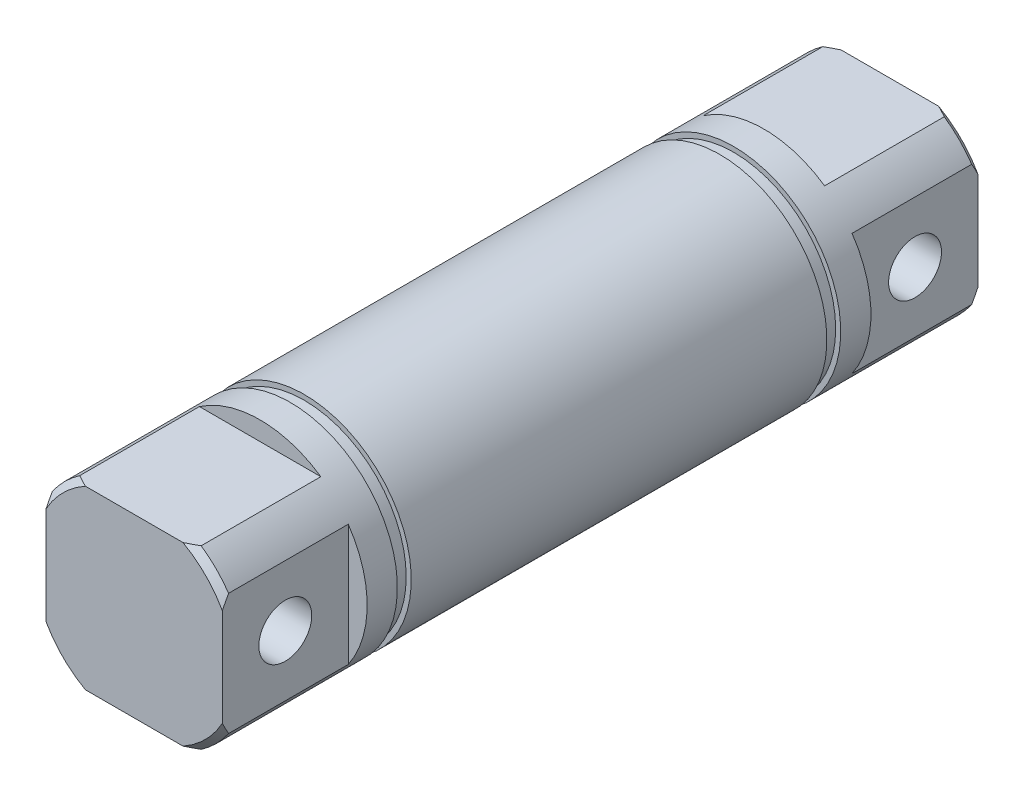
from build123d import *

# Parameters (mm, degrees)
SKETCH_1_R           = 8.5
EXTRUDE_1_DEPTH      = 30
SKETCH_4_OUTSIDE_W   = 31.928
SKETCH_4_OUTSIDE_H   = 31.928
SKETCH_4_OUTSIDE_W_2 = 14
SKETCH_4_OUTSIDE_H_2 = 14
CUT_EXTRUDE_1_DEPTH  = 10
HOLE_WIZARD_M5_1_D   = 4.2
CHAMFER_1_SIZE       = 0.5
SKETCH_7_W           = 0.4
SKETCH_7_H           = 1.1


with BuildPart() as part:
    # 草图1 → 凸台-拉伸1 (new, symmetric)
    with BuildSketch(Plane.XY):
        Circle(SKETCH_1_R)
    extrude(amount=EXTRUDE_1_DEPTH, both=True)

    # 草图4 outside → 切除-拉伸1 (cut)
    with BuildSketch(Plane.XY.offset(30)):
        Rectangle(SKETCH_4_OUTSIDE_W, SKETCH_4_OUTSIDE_H)
        Rectangle(SKETCH_4_OUTSIDE_W_2, SKETCH_4_OUTSIDE_H_2, mode=Mode.SUBTRACT)
    cut_extrude_1 = extrude(amount=-CUT_EXTRUDE_1_DEPTH, mode=Mode.SUBTRACT)

    # M5 螺纹孔1 (through all)
    with Locations(Plane(origin=(7, 0, 0), x_dir=(0, 0, -1), z_dir=(1, 0, 0))):
        with Locations((-25, 0)):
            hole_wizard_m5_1 = Hole(HOLE_WIZARD_M5_1_D / 2)

    # 镜向1: 切除-拉伸1, M5 螺纹孔1 across plane
    add(cut_extrude_1.mirror(Plane.XY), mode=Mode.SUBTRACT)
    add(hole_wizard_m5_1.mirror(Plane.XY), mode=Mode.SUBTRACT)

    # 倒角1
    chamfer_1_edges = [part.edges().sort_by_distance(p)[0] for p in [
        (6.01040764, 6.01040764, -30),
        (6.01040764, 6.01040764, 30),
        (-6.01040764, 6.01040764, 30),
        (-6.01040764, 6.01040764, -30),
        (-6.01040764, -6.01040764, -30),
        (6.01040764, -6.01040764, -30),
        (-6.01040764, -6.01040764, 30),
        (6.01040764, -6.01040764, 30),
    ]]
    chamfer(chamfer_1_edges, length=CHAMFER_1_SIZE)

    # 草图7 → 切除-旋转1 (revolve, cut)
    with BuildSketch(Plane(origin=(0, 0, 0), x_dir=(1, 0, 0), z_dir=(0, 1, 0)), mode=Mode.PRIVATE) as cut_revolve_1_sk:
        with Locations((8.3, 17.05)):
            Rectangle(SKETCH_7_W, SKETCH_7_H)
    cut_revolve_1 = revolve(cut_revolve_1_sk.sketch.rotate(Axis((0, 0, -14.7653446), (0, 0, 1)), 180), axis=Axis((0, 0, -14.7653446), (0, 0, 1)), mode=Mode.SUBTRACT)

    # 镜向2: 切除-旋转1 across plane
    add(cut_revolve_1.mirror(Plane.XY), mode=Mode.SUBTRACT)


solid = part.part
